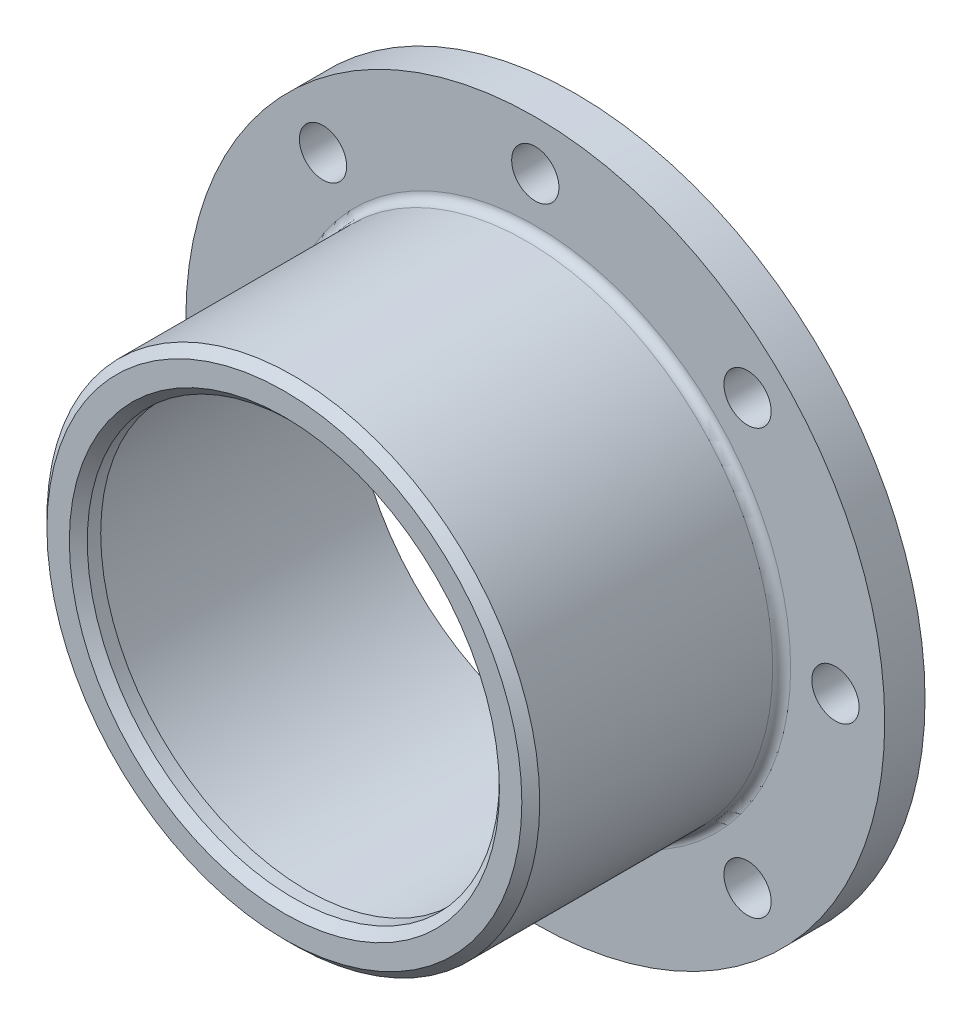
from build123d import *

# Parameters (mm, degrees)
SKETCH1_R           = 78
BOSS_EXTRUDE1_DEPTH = 9
SKETCH2_R           = 55
BOSS_EXTRUDE2_DEPTH = 56
SKETCH3_R           = 50
CUT_EXTRUDE2_DEPTH  = 60
SKETCH4_R           = 46
CUT_EXTRUDE3_DEPTH  = 129.035151423
SKETCH5_R           = 5.275
CUT_EXTRUDE4_DEPTH  = 129.035151423
CIRPATTERN1_COUNT   = 8
CHAMFER1_SIZE       = 2
FILLET1_R           = 2


with BuildPart() as part:
    # Sketch1 → Boss-Extrude1 (new body)
    with BuildSketch(Plane.XY):
        Circle(SKETCH1_R)
    extrude(amount=BOSS_EXTRUDE1_DEPTH)

    # Sketch2 → Boss-Extrude2 (add)
    with BuildSketch(Plane.XY.offset(9)):
        Circle(SKETCH2_R)
    extrude(amount=BOSS_EXTRUDE2_DEPTH)

    # Sketch3 → Cut-Extrude2 (cut)
    with BuildSketch(Plane(origin=(0, 0, 0), x_dir=(-1, 0, 0), z_dir=(0, 0, -1))):
        Circle(SKETCH3_R)
    extrude(amount=-CUT_EXTRUDE2_DEPTH, mode=Mode.SUBTRACT)

    # Sketch4 → Cut-Extrude3 (cut, through all)
    with BuildSketch(Plane.XY.offset(65)):
        Circle(SKETCH4_R)
    extrude(amount=-CUT_EXTRUDE3_DEPTH, mode=Mode.SUBTRACT)

    # Sketch5 → Cut-Extrude4 (cut, through all)
    with BuildSketch(Plane(origin=(0, 0, 0), x_dir=(-1, 0, 0), z_dir=(0, 0, -1))):
        with Locations((0, 67)):
            Circle(SKETCH5_R)
    cut_extrude4 = extrude(amount=-CUT_EXTRUDE4_DEPTH, mode=Mode.SUBTRACT)

    # CirPattern1: Cut-Extrude4 ×8 about axis
    cirpattern1_axis = Axis((0, 0, 0), (0, 0, 1))
    for i in range(1, CIRPATTERN1_COUNT):
        add(cut_extrude4.rotate(cirpattern1_axis, i * 360 / CIRPATTERN1_COUNT), mode=Mode.SUBTRACT)

    # Chamfer1
    chamfer1_edges = [part.edges().sort_by_distance(p)[0] for p in [
        (-46, 0, 65),
        (-55, 0, 65),
    ]]
    chamfer(chamfer1_edges, length=CHAMFER1_SIZE)

    # Fillet1
    fillet1_edges = [part.edges().sort_by_distance(p)[0] for p in [
        (-55, 0, 9),
    ]]
    fillet(fillet1_edges, radius=FILLET1_R)


solid = part.part
